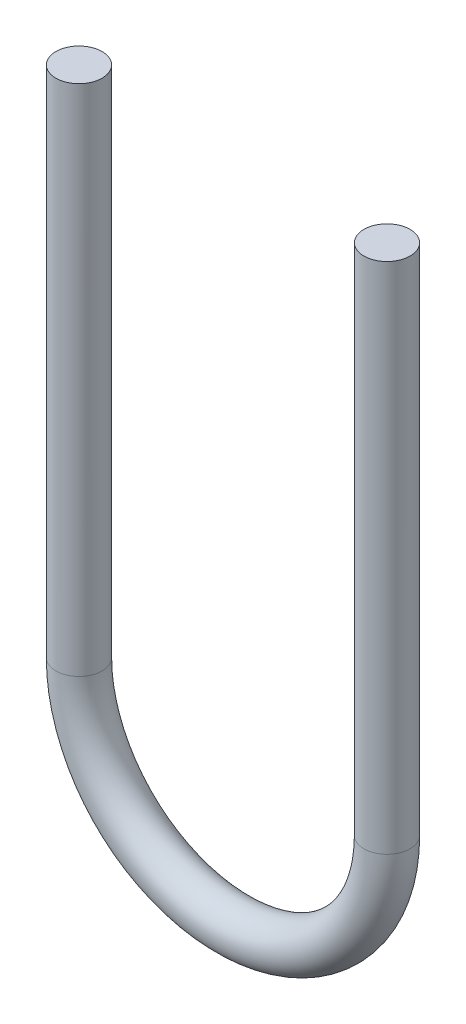
from build123d import *

# Parameters (mm, degrees)
SKETCH2_R = 4.5


with BuildPart() as part:
    # Sweep1: sweep along a path in Sketch1
    with BuildLine(Plane.XY) as sweep1_path:
        Line((60, 0), (60, -100))
        ThreePointArc((60, -100), (30, -130), (0, -100))
        Line((0, -100), (0, 0))
    # Sketch2 → Sweep1 (sweep)
    with BuildSketch(Plane(origin=(0, 0, 0), x_dir=(1, 0, 0), z_dir=(0, 1, 0))):
        Circle(SKETCH2_R)
    sweep(path=sweep1_path.line)


solid = part.part
